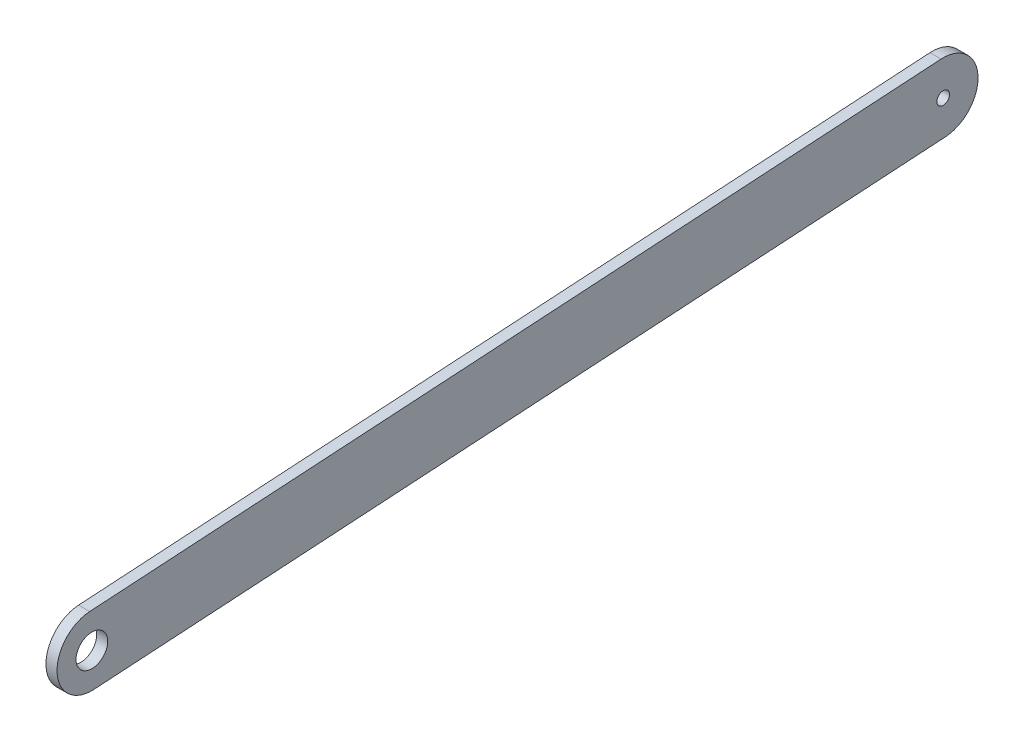
SolidWorks part; units mm, degrees
ref_plane "前视基准面" through (0, 0, 0) normal (0, 0, 1) x (1, 0, 0)
ref_plane "上视基准面" through (0, 0, 0) normal (0, 1, 0) x (1, 0, 0)
ref_plane "右视基准面" through (0, 0, 0) normal (1, 0, 0) x (0, 0, -1)
other "Configuration Table"
sketch "草图1" plane through (797.5975, 0, 0) normal (1, 0, 0) x (0, 0, -1)
  line L5 (-187.2657, -33.2875) -> (350, 0) construction
  line L8 (-188.6261, -11.3296) -> (348.6396, 21.9579)
  line L9 (-185.9052, -55.2454) -> (351.3604, -21.9579)
  circle A5 centre (-187.2657, -33.2875) radius 16 construction
  circle A9 centre (350, 0) radius 4
  circle A10 centre (-187.2657, -33.2875) radius 16 construction
  arc A13 (-177.7379, -36.324) -> (-184.1271, -42.7822) centre (-187.2657, -33.2875) ccw construction
  arc A14 (-177.7379, -36.324) -> (-184.1271, -42.7822) centre (-187.2657, -33.2875) ccw construction
  circle A15 centre (-187.2657, -33.2875) radius 10
  arc A16 (-188.6261, -11.3296) -> (-185.9052, -55.2454) centre (-187.2657, -33.2875) ccw
  arc A17 (351.3604, -21.9579) -> (348.6396, 21.9579) centre (350, 0) ccw
  point P3 (81.3672, -16.6437)
  dimension "D1" = 22
  dimension "D3" = 8
  dimension "D4" = 537.2657
  dimension "D2" = 20
extrude "凸台-拉伸1" add sketch "草图1" against normal blind 7
